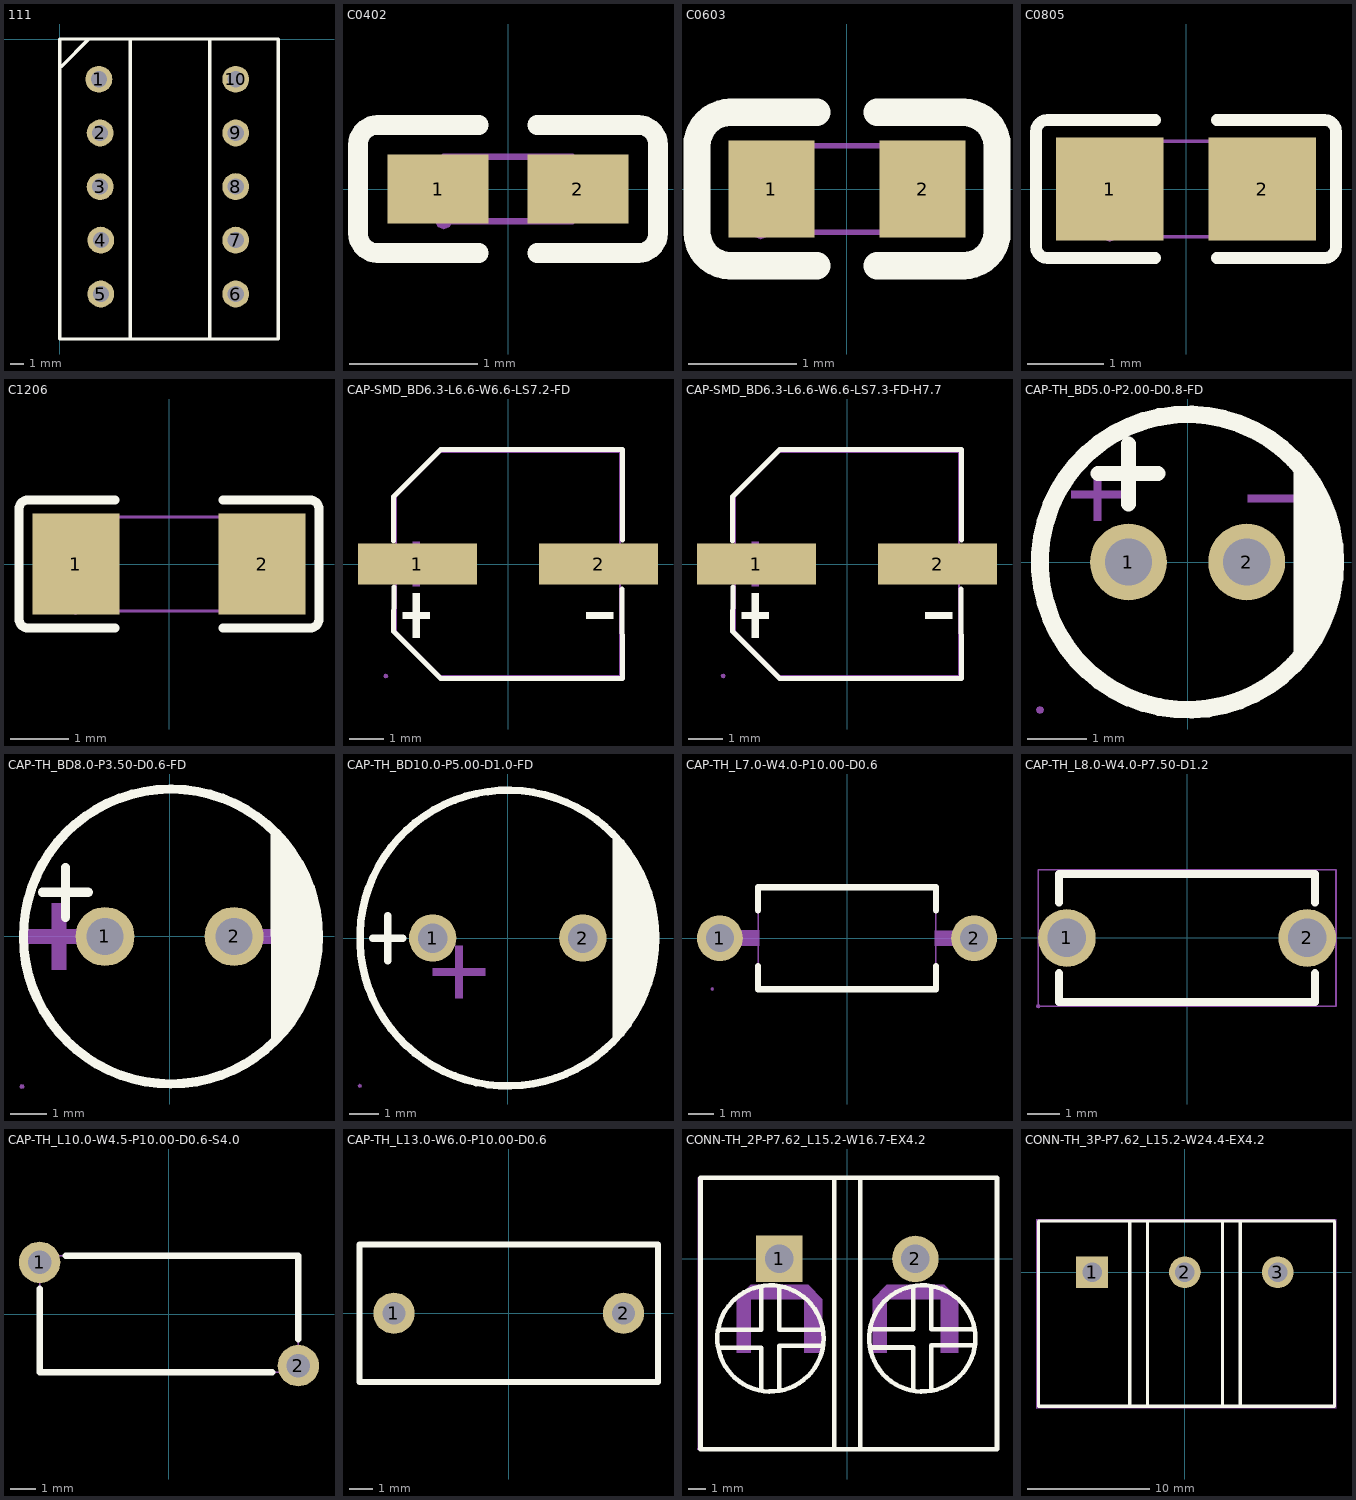
[diagram p0: the footprints below, top view; thin cyan lines are the x and y axes]
# Altium footprint library MISC84429-11.PcbLib: 64 footprints (part 1 of 4)
Each footprint in its own frame and in the unit in brackets; x right, y up, seen from the top. Pads: shape width x height; smd on the part's side, far side on the other; paste and mask are expansions set on the pad; w line width, h text height; cw(c..) or ccw(c..) is an arc to the next point about the centre after c.

## 111 [mm]
pads (10):
  round 2 hole 1.2 paste+0 mask-0.349: 1(2.901,-3) 2(3,-7) 3(3,-11.001) 4(3.048,-14.989) 5(3.048,-18.999) 6(13.099,-18.999) 7(13.099,-14.989) 8(13.099,-11.001) 9(13.099,-7) 10(13.099,-3)
Top Overlay:
  lines w0.254: 0.127,-2.018 2.159,0 ; 5.255,-22.352 5.255,0 ; 11.176,-22.352 11.176,0 ; 0,-22.352 0,0 16.256,0 16.256,-22.352 0,-22.352

## C0402 [mm]
pads (2):
  rect 0.79x0.54 smd paste-100 mask+0.051: 1(-0.545,0) 2(0.545,0)
Top Overlay:
  lines w0.152: -0.226,-0.499 -1.016,-0.499 cw(c-1.016,-0.346) -1.169,-0.346 -1.169,0.346 cw(c-1.016,0.346) -1.016,0.499 -0.226,0.499 ; 0.226,-0.499 1.016,-0.499 ccw(c1.016,-0.346) 1.169,-0.346 1.169,0.346 ccw(c1.016,0.346) 1.016,0.499 0.226,0.499
Top Paste:
  region: -0.18,0.225 -0.18,-0.225 -0.25,-0.275 -0.73,-0.275 -0.78,-0.225 -0.78,0.225 -0.73,0.275 -0.25,0.275
  region: 0.78,0.225 0.78,-0.225 0.73,-0.275 0.25,-0.275 0.18,-0.225 0.18,0.225 0.25,0.275 0.73,0.275
Mechanical 2:
  region: -0.435,-0.25 -0.454,-0.296 -0.5,-0.315 -0.546,-0.296 -0.565,-0.25 -0.546,-0.204 -0.5,-0.185 -0.454,-0.204
  region: -0.5,-0.25 -0.5,0.25 -0.25,0.25 -0.25,-0.25
  region: 0.5,-0.25 0.5,0.25 0.25,0.25 0.25,-0.25
  lines w0.051: -0.5,-0.25 -0.5,0.25 0.5,0.25 0.5,-0.25 -0.5,-0.25

## C0603 [mm]
pads (2):
  rect 0.8x0.9 smd: 1(-0.7,0) 2(0.7,0)
Top Overlay:
  lines w0.254: -1.08,-0.71 -0.28,-0.71 ; -1.08,0.71 -0.28,0.71 ; -1.08,-0.71 cw(c-1.08,-0.4) -1.39,-0.4 -1.39,0.4 cw(c-1.08,0.4) -1.08,0.71 ; 0.28,-0.71 1.08,-0.71 ccw(c1.08,-0.4) 1.39,-0.4 1.39,0.4 ccw(c1.08,0.4) 1.08,0.71 0.28,0.71
Mechanical 2:
  region: -0.735,-0.4 -0.754,-0.446 -0.8,-0.465 -0.846,-0.446 -0.865,-0.4 -0.846,-0.354 -0.8,-0.335 -0.754,-0.354
  region: -0.8,-0.4 -0.8,0.4 -0.5,0.4 -0.5,-0.4
  region: 0.8,-0.4 0.8,0.4 0.5,0.4 0.5,-0.4
  lines w0.051: -0.8,-0.4 -0.8,0.4 0.8,0.4 0.8,-0.4 -0.8,-0.4

## C0805 [mm]
pads (2):
  rect 1.41x1.35 smd paste-100 mask+0.051: 1(-1,0) 2(1,0)
Top Overlay:
  lines w0.152: -0.401,-0.904 -1.811,-0.904 cw(c-1.811,-0.751) -1.964,-0.751 -1.964,0.751 cw(c-1.811,0.751) -1.811,0.904 -0.401,0.904 ; 0.401,-0.904 1.811,-0.904 ccw(c1.811,-0.751) 1.964,-0.751 1.964,0.751 ccw(c1.811,0.751) 1.811,0.904 0.401,0.904
Top Paste:
  region: -1.705,-0.64 -1.705,0.64 -1.655,0.69 -0.505,0.69 -0.455,0.64 -0.45,0.23 -0.9,0.23 -0.9,-0.22 -0.46,-0.22 -0.455,-0.64 -0.505,-0.69 -1.655,-0.69
  region: 1.705,0.64 1.705,-0.64 1.655,-0.69 0.505,-0.69 0.455,-0.64 0.45,-0.23 0.9,-0.23 0.9,0.22 0.46,0.22 0.455,0.64 0.505,0.69 1.655,0.69
Mechanical 2:
  region: -0.935,-0.625 -0.954,-0.671 -1,-0.69 -1.046,-0.671 -1.065,-0.625 -1.046,-0.579 -1,-0.56 -0.954,-0.579
  region: -1,-0.625 -1,0.625 -0.5,0.625 -0.5,-0.625
  region: 1,0.625 1,-0.625 0.5,-0.625 0.5,0.625
  lines w0.051: -1,-0.625 -1,0.625 1,0.625 1,-0.625 -1,-0.625

## C1206 [mm]
pads (2):
  rect 1.485x1.728 smd paste-100 mask+0.051: 1(-1.593,0) 2(1.593,0)
Top Overlay:
  lines w0.152: -0.926,-1.093 -2.411,-1.093 cw(c-2.411,-0.94) -2.564,-0.94 -2.564,0.94 cw(c-2.411,0.94) -2.411,1.093 -0.926,1.093 ; 0.926,-1.093 2.411,-1.093 ccw(c2.411,-0.94) 2.564,-0.94 2.564,0.94 ccw(c2.411,0.94) 2.411,1.093 0.926,1.093
Top Paste:
  region: 0.85,-0.764 0.85,-0.394 0.95,-0.294 1.255,-0.294 1.355,-0.194 1.355,0.194 1.255,0.294 0.95,0.294 0.85,0.394 0.85,0.764 0.95,0.864 2.235,0.864 2.335,0.764 2.335,-0.764 2.235,-0.864 0.95,-0.864
  region: -0.85,-0.764 -0.85,-0.394 -0.95,-0.294 -1.255,-0.294 -1.355,-0.194 -1.355,0.194 -1.255,0.294 -0.95,0.294 -0.85,0.394 -0.85,0.764 -0.95,0.864 -2.235,0.864 -2.335,0.764 -2.335,-0.764 -2.235,-0.864 -0.95,-0.864
Mechanical 2:
  region: -1.535,-0.8 -1.554,-0.846 -1.6,-0.865 -1.646,-0.846 -1.665,-0.8 -1.646,-0.754 -1.6,-0.735 -1.554,-0.754
  region: -1.6,-0.8 -1.6,0.8 -1.1,0.8 -1.1,-0.8
  region: 1.6,-0.8 1.6,0.8 1.1,0.8 1.1,-0.8
  lines w0.051: -1.6,-0.8 -1.6,0.8 1.6,0.8 1.6,-0.8 -1.6,-0.8

## CAP-SMD_BD6.3-L6.6-W6.6-LS7.2-FD [mm]
pads (2):
  rect 3.5x1.2 smd: 1(-2.67,0) 2(2.67,0)
Top Overlay:
  region: -2.805,-0.858 -2.805,-2.178 -2.607,-2.178 -2.607,-0.858
  region: -3.102,-1.419 -3.102,-1.617 -2.31,-1.617 -2.31,-1.419
  region: 3.102,-1.419 3.102,-1.617 2.31,-1.617 2.31,-1.419
  lines w0.152: -3.376,0.686 -3.376,1.98 -1.98,3.376 3.376,3.376 3.369,0.708 ; -3.362,-0.686 -3.376,-1.981 -1.981,-3.376 3.376,-3.376 3.356,-0.739
Mechanical 1:
  region: -2.805,0.66 -2.805,-0.66 -2.607,-0.66 -2.607,0.66
  region: -3.102,0.099 -3.102,-0.099 -2.31,-0.099 -2.31,0.099
  region: 3.102,0.099 3.102,-0.099 2.31,-0.099 2.31,0.099
Mechanical 2:
  region: -3.535,-3.3 -3.554,-3.346 -3.6,-3.365 -3.646,-3.346 -3.665,-3.3 -3.646,-3.254 -3.6,-3.235 -3.554,-3.254
  region: 0.95,0.35 3.6,0.35 3.6,-0.35 0.95,-0.35
  region: -3.6,0.35 -0.95,0.35 -0.95,-0.35 -3.6,-0.35
  lines w0.051: -3.3,-1.98 -1.98,-3.3 3.3,-3.3 3.3,3.3 -1.98,3.3 -3.3,1.98 -3.3,-1.98

## CAP-SMD_BD6.3-L6.6-W6.6-LS7.3-FD-H7.7 [mm]
pads (2):
  rect 3.5x1.2 smd: 1(-2.67,0) 2(2.67,0)
Top Overlay:
  region: 3.102,-1.419 3.102,-1.617 2.31,-1.617 2.31,-1.419
  region: -3.102,-1.419 -3.102,-1.617 -2.31,-1.617 -2.31,-1.419
  region: -2.805,-0.858 -2.805,-2.178 -2.607,-2.178 -2.607,-0.858
  lines w0.152: -3.376,0.686 -3.376,1.98 -1.98,3.376 3.376,3.376 3.369,0.708 ; -3.362,-0.686 -3.376,-1.981 -1.981,-3.376 3.376,-3.376 3.356,-0.739
Mechanical 1:
  region: 3.102,0.099 3.102,-0.099 2.31,-0.099 2.31,0.099
  region: -3.102,0.099 -3.102,-0.099 -2.31,-0.099 -2.31,0.099
  region: -2.805,0.66 -2.805,-0.66 -2.607,-0.66 -2.607,0.66
Mechanical 2:
  region: -3.587,-3.3 -3.606,-3.346 -3.652,-3.365 -3.697,-3.346 -3.716,-3.3 -3.697,-3.254 -3.652,-3.235 -3.606,-3.254
  region: -3.652,0.35 -1.002,0.35 -1.002,-0.35 -3.652,-0.35
  region: 0.999,0.35 3.649,0.35 3.649,-0.35 0.999,-0.35
  lines w0.051: -3.3,-1.98 -1.98,-3.3 3.3,-3.3 3.3,3.3 -1.98,3.3 -3.3,1.98 -3.3,-1.98

## CAP-TH_BD5.0-P2.00-D0.8-FD [mm]
pads (2):
  round 1.3 hole 0.8: 1(-1,0) 2(1,0)
Top Overlay:
  circle w0.3: c0,0 r2.5
  region: 1.799,1.656 1.839,1.622 2.124,1.275 2.336,0.878 2.467,0.448 2.511,0 2.467,-0.448 2.336,-0.878 2.124,-1.275 1.839,-1.622 1.799,-1.656 1.794,-1.651
  lines w0.254: -1.516,1.5 -0.5,1.5 ; -1,0.984 -1,2
Mechanical 1:
  region: -1.969,1.206 -1.08,1.206 -1.08,1.079 -1.969,1.079
  region: -1.588,0.699 -1.588,1.587 -1.461,1.587 -1.46,0.699
  region: 1.016,1.143 1.905,1.143 1.905,1.016 1.016,1.016
Mechanical 2:
  region: -2.435,-2.5 -2.454,-2.546 -2.5,-2.565 -2.546,-2.546 -2.565,-2.5 -2.546,-2.454 -2.5,-2.435 -2.454,-2.454
  region: -0.694,0 -0.717,-0.117 -0.784,-0.216 -0.883,-0.283 -1,-0.306 -1.117,-0.283 -1.216,-0.216 -1.283,-0.117 -1.306,0 -1.283,0.117 -1.216,0.216 -1.117,0.283 -1,0.306 -0.883,0.283 -0.784,0.216 -0.717,0.117
  region: 1.306,0 1.283,-0.117 1.216,-0.216 1.117,-0.283 1,-0.306 0.883,-0.283 0.784,-0.216 0.717,-0.117 0.694,0 0.717,0.117 0.784,0.216 0.883,0.283 1,0.306 1.117,0.283 1.216,0.216 1.283,0.117
  lines w0.051: 0,-2.5 cw(c0,0) -2.5,0 cw(c0,0) 0,2.5 cw(c0,0) 2.5,0 ; 0,-2.5 ccw(c0,0) 2.5,0 ; 0,-2.5 0,-2.5 ; 2.5,0 2.5,0

## CAP-TH_BD8.0-P3.50-D0.6-FD [mm]
pads (2):
  round 1.6 hole 1: 1(-1.75,0) 2(1.75,0)
Top Overlay:
  region: 2.753,-3.003 3.059,-2.654 3.375,-2.18 3.628,-1.668 3.811,-1.128 3.922,-0.569 3.959,0 3.922,0.569 3.811,1.128 3.628,1.668 3.375,2.18 3.059,2.654 2.753,3.003 2.75,3
  lines w0.254: -3.445,1.2 -2.2,1.2 ; -2.822,0.527 -2.822,1.873 ; 0.003,4 ccw(c0.038,0.001) 0.074,4
Mechanical 1:
  region: 2.1,0.2 2.1,-0.2 3.9,-0.2 3.9,0.2
  region: -3.9,0.2 -3.9,-0.2 -2.1,-0.2 -2.1,0.2
  region: -3.2,-0.9 -2.8,-0.9 -2.8,0.9 -3.2,0.9
Mechanical 2:
  region: -3.936,-4.072 -3.955,-4.118 -4.001,-4.137 -4.047,-4.118 -4.066,-4.072 -4.047,-4.026 -4.001,-4.007 -3.955,-4.026
  region: 2.056,0 2.033,-0.117 1.966,-0.216 1.867,-0.283 1.75,-0.306 1.633,-0.283 1.534,-0.216 1.467,-0.117 1.444,0 1.467,0.117 1.534,0.216 1.633,0.283 1.75,0.306 1.867,0.283 1.966,0.216 2.033,0.117
  region: -1.444,0 -1.467,-0.117 -1.534,-0.216 -1.633,-0.283 -1.75,-0.306 -1.867,-0.283 -1.966,-0.216 -2.033,-0.117 -2.056,0 -2.033,0.117 -1.966,0.216 -1.867,0.283 -1.75,0.306 -1.633,0.283 -1.534,0.216 -1.467,0.117
  lines w0.051: -0.003,-4.072 cw(c-0.001,-0.072) 0,-4.072 -0.003,-4.072

## CAP-TH_BD10.0-P5.00-D1.0-FD [mm]
pads (2):
  round 1.6 hole 1: 1(-2.54,0) 2(2.54,0)
Top Overlay:
  circle w0.254: c0,0 r5
  region: 3.556,3.556 3.556,-3.556 4.318,-2.54 4.826,-1.016 5.08,0.508 4.826,1.524
  lines w0.254: -4.572,0 -3.556,0 ; -4.064,-0.762 -4.064,0.762
Mechanical 1:
  region: -2.54,-1.016 -0.762,-1.016 -0.762,-1.27 -2.54,-1.27
  region: -1.778,-2.032 -1.524,-2.032 -1.524,-0.254 -1.778,-0.254
Mechanical 2:
  region: -4.935,-5 -4.954,-5.046 -5,-5.065 -5.046,-5.046 -5.065,-5 -5.046,-4.954 -5,-4.935 -4.954,-4.954
  region: 2.846,0 2.823,-0.117 2.756,-0.216 2.657,-0.283 2.54,-0.306 2.423,-0.283 2.324,-0.216 2.257,-0.117 2.234,0 2.257,0.117 2.324,0.216 2.423,0.283 2.54,0.306 2.657,0.283 2.756,0.216 2.823,0.117
  region: -2.234,0 -2.257,-0.117 -2.324,-0.216 -2.423,-0.283 -2.54,-0.306 -2.657,-0.283 -2.756,-0.216 -2.823,-0.117 -2.846,0 -2.823,0.117 -2.756,0.216 -2.657,0.283 -2.54,0.306 -2.423,0.283 -2.324,0.216 -2.257,0.117
  lines w0.051: -5,0 cw(c0,0) 5,0 cw(c0,0) -5,0

## CAP-TH_L7.0-W4.0-P10.00-D0.6 [mm]
pads (2):
  round 1.8 hole 1.1: 1(-5,0) 2(5,0)
Top Overlay:
  lines w0.254: -3.5,-1.103 -3.5,-2 3.5,-2 3.5,-1.103 ; -3.5,1.103 -3.5,2 3.5,2 3.5,1.103
Mechanical 2:
  region: -5.237,-2 -5.256,-2.046 -5.301,-2.065 -5.347,-2.046 -5.366,-2 -5.347,-1.954 -5.301,-1.935 -5.256,-1.954
  region: -4.694,0 -4.717,-0.117 -4.784,-0.216 -4.883,-0.283 -5,-0.306 -5.117,-0.283 -5.216,-0.216 -5.283,-0.117 -5.306,0 -5.283,0.117 -5.216,0.216 -5.117,0.283 -5,0.306 -4.883,0.283 -4.784,0.216 -4.717,0.117
  region: 5.306,0 5.283,-0.117 5.216,-0.216 5.117,-0.283 5,-0.306 4.883,-0.283 4.784,-0.216 4.717,-0.117 4.694,0 4.717,0.117 4.784,0.216 4.883,0.283 5,0.306 5.117,0.283 5.216,0.216 5.283,0.117
  region: -3.452,-0.295 -5.302,-0.295 -5.302,0.305 -3.452,0.305
  region: 5.3,-0.299 3.45,-0.299 3.45,0.301 5.3,0.301
  lines w0.051: -3.5,-2 -3.5,2 3.5,2 3.5,-2 -3.5,-2

## CAP-TH_L8.0-W4.0-P7.50-D1.2 [mm]
pads (2):
  round 1.8 hole 1.2: 1(-3.75,0) 2(3.75,0)
Top Overlay:
  lines w0.254: -4,-1.103 -4,-2 4,-2 4,-1.103 ; -4,1.103 -4,2 4,2 4,1.103
Mechanical 2:
  region: -3.24,0 -3.279,-0.195 -3.39,-0.36 -3.555,-0.471 -3.75,-0.51 -3.945,-0.471 -4.111,-0.36 -4.221,-0.195 -4.26,0 -4.221,0.195 -4.111,0.36 -3.945,0.471 -3.75,0.51 -3.555,0.471 -3.39,0.36 -3.279,0.195
  region: 4.26,0 4.221,-0.195 4.111,-0.36 3.945,-0.471 3.75,-0.51 3.555,-0.471 3.39,-0.36 3.279,-0.195 3.24,0 3.279,0.195 3.39,0.36 3.555,0.471 3.75,0.51 3.945,0.471 4.111,0.36 4.221,0.195
  region: -4.585,-2.127 -4.604,-2.173 -4.65,-2.192 -4.696,-2.173 -4.715,-2.127 -4.696,-2.081 -4.65,-2.062 -4.604,-2.081
  lines w0.051: -4.65,-2.127 4.65,-2.127 4.65,2.127 -4.65,2.127 -4.65,-2.127

## CAP-TH_L10.0-W4.5-P10.00-D0.6-S4.0 [mm]
pads (2):
  round 1.6 hole 0.9: 1(-5,2) 2(5,-2)
Top Overlay:
  lines w0.254: -5,0.469 -5,0.969 -5,-2.25 4,-2.25 ; -4,2.25 5,2.25 5,-0.469 5,-0.969
Mechanical 2:
  region: -5.21,2.275 -5.229,2.229 -5.275,2.21 -5.321,2.229 -5.34,2.275 -5.321,2.321 -5.275,2.34 -5.229,2.321
  region: 5.28,-2 5.259,-2.107 5.198,-2.198 5.107,-2.259 5,-2.28 4.893,-2.259 4.802,-2.198 4.741,-2.107 4.72,-2 4.741,-1.893 4.802,-1.802 4.893,-1.741 5,-1.72 5.107,-1.741 5.198,-1.802 5.259,-1.893
  region: -4.72,2 -4.741,1.893 -4.802,1.802 -4.893,1.741 -5,1.72 -5.107,1.741 -5.198,1.802 -5.259,1.893 -5.28,2 -5.259,2.107 -5.198,2.198 -5.107,2.259 -5,2.28 -4.893,2.259 -4.802,2.198 -4.741,2.107
  lines w0.051: -5,-2.25 -5,2.25 5,2.25 5,-2.25 -5,-2.25

## CAP-TH_L13.0-W6.0-P10.00-D0.6 [mm]
pads (2):
  round 1.8 hole 1: 1(-5,0) 2(5,0)
Top Overlay:
  lines w0.254: -6.5,-3 6.5,-3 6.5,3 -6.5,3 -6.5,-3
Mechanical 2:
  region: -6.435,-3 -6.454,-3.046 -6.5,-3.065 -6.546,-3.046 -6.565,-3 -6.546,-2.954 -6.5,-2.935 -6.454,-2.954
  region: 5.306,0 5.283,-0.117 5.216,-0.216 5.117,-0.283 5,-0.306 4.883,-0.283 4.784,-0.216 4.717,-0.117 4.694,0 4.717,0.117 4.784,0.216 4.883,0.283 5,0.306 5.117,0.283 5.216,0.216 5.283,0.117
  region: -4.694,0 -4.717,-0.117 -4.784,-0.216 -4.883,-0.283 -5,-0.306 -5.117,-0.283 -5.216,-0.216 -5.283,-0.117 -5.306,0 -5.283,0.117 -5.216,0.216 -5.117,0.283 -5,0.306 -4.883,0.283 -4.784,0.216 -4.717,0.117
  lines w0.051: -6.5,-3 -6.5,3 6.5,3 6.5,-3 -6.5,-3

## CONN-TH_2P-P7.62_L15.2-W16.7-EX4.2 [mm]
pads (2):
  rect 2.6x2.6 hole 1.6: 1(-3.81,0)
  round 2.6 hole 1.6: 2(3.81,0)
Top Overlay:
  circle w0.254: c4.2,-4.45 r2.973
  circle w0.254: c-4.3,-4.45 r2.973
  lines w0.254: -7.229,-4.979 -4.816,-4.979 -4.816,-7.265 ; -7.229,-3.963 -4.816,-3.963 -4.816,-1.55 ; -3.8,-7.265 -3.8,-4.852 -1.387,-4.852 ; -3.8,-1.55 -3.8,-3.963 -1.387,-3.963 ; 1.279,-4.958 3.692,-4.958 3.692,-7.244 ; 1.279,-3.942 3.692,-3.942 3.692,-1.529 ; 4.708,-7.244 4.708,-4.831 7.121,-4.831 ; 4.708,-1.529 4.708,-3.942 7.121,-3.942 ; -8.22,-10.65 8.38,-10.65 8.38,4.55 -8.22,4.55 -8.22,-10.65 ; -0.72,-10.65 0.73,-10.65 0.73,4.55 -0.72,4.55 -0.72,-10.65
Mechanical 1:
  region: -6.2,-5.25 -6.2,-2.25 -5.4,-2.25 -5.4,-5.25
  region: -6.2,-2.25 -5.4,-1.45 -2.2,-1.45 -1.4,-2.25
  region: -2.4,-5.25 -1.4,-5.25 -1.4,-2.25 -2.4,-2.25
  region: 1.42,-5.25 1.42,-2.25 2.22,-2.25 2.22,-5.25
  region: 1.42,-2.25 2.22,-1.45 5.42,-1.45 6.22,-2.25
  region: 5.22,-5.25 6.22,-5.25 6.22,-2.25 5.22,-2.25
Mechanical 2:
  region: -8.285,-10.65 -8.304,-10.696 -8.35,-10.715 -8.396,-10.696 -8.415,-10.65 -8.396,-10.604 -8.35,-10.585 -8.304,-10.604
  region: -4.41,0.4 -3.21,0.4 -3.21,-0.4 -4.41,-0.4
  region: 3.21,0.4 4.41,0.4 4.41,-0.4 3.21,-0.4
  lines w0.051: -8.35,-10.65 -8.35,4.55 8.35,4.55 8.35,-10.65 -8.35,-10.65

## CONN-TH_3P-P7.62_L15.2-W24.4-EX4.2 [mm]
pads (3):
  rect 2.6x2.6 hole 1.6: 1(-7.62,0)
  round 2.6 hole 1.6: 2(0,0) 3(7.62,0)
Top Overlay:
  lines w0.254: -12.03,-11 12.27,-11 12.27,4.2 -12.03,4.2 -12.03,-11 ; -4.53,-11 -3.08,-11 -3.08,4.2 -4.53,4.2 -4.53,-11 ; 3.09,-11 4.54,-11 4.54,4.2 3.09,4.2 3.09,-11
Mechanical 2:
  region: -6.914,0 -6.938,-0.183 -7.009,-0.353 -7.121,-0.499 -7.267,-0.611 -7.437,-0.682 -7.62,-0.706 -7.803,-0.682 -7.973,-0.611 -8.119,-0.499 -8.231,-0.353 -8.302,-0.183 -8.326,0 -8.302,0.183 -8.231,0.353 -8.119,0.499 -7.973,0.611 -7.803,0.682 -7.62,0.706 -7.437,0.682 -7.267,0.611 -7.121,0.499 -7.009,0.353 -6.938,0.183
  region: 0.706,0 0.682,-0.183 0.611,-0.353 0.499,-0.499 0.353,-0.611 0.183,-0.682 0,-0.706 -0.183,-0.682 -0.353,-0.611 -0.499,-0.499 -0.611,-0.353 -0.682,-0.183 -0.706,0 -0.682,0.183 -0.611,0.353 -0.499,0.499 -0.353,0.611 -0.183,0.682 0,0.706 0.183,0.682 0.353,0.611 0.499,0.499 0.611,0.353 0.682,0.183
  region: 8.326,0 8.302,-0.183 8.231,-0.353 8.119,-0.499 7.973,-0.611 7.803,-0.682 7.62,-0.706 7.437,-0.682 7.267,-0.611 7.121,-0.499 7.009,-0.353 6.938,-0.183 6.914,0 6.938,0.183 7.009,0.353 7.121,0.499 7.267,0.611 7.437,0.682 7.62,0.706 7.803,0.682 7.973,0.611 8.119,0.499 8.231,0.353 8.302,0.183
  region: -12.092,-11.127 -12.111,-11.173 -12.157,-11.192 -12.203,-11.173 -12.222,-11.127 -12.203,-11.081 -12.157,-11.062 -12.111,-11.081
  lines w0.051: -12.157,-11.127 12.397,-11.127 12.397,4.327 -12.157,4.327 -12.157,-11.127